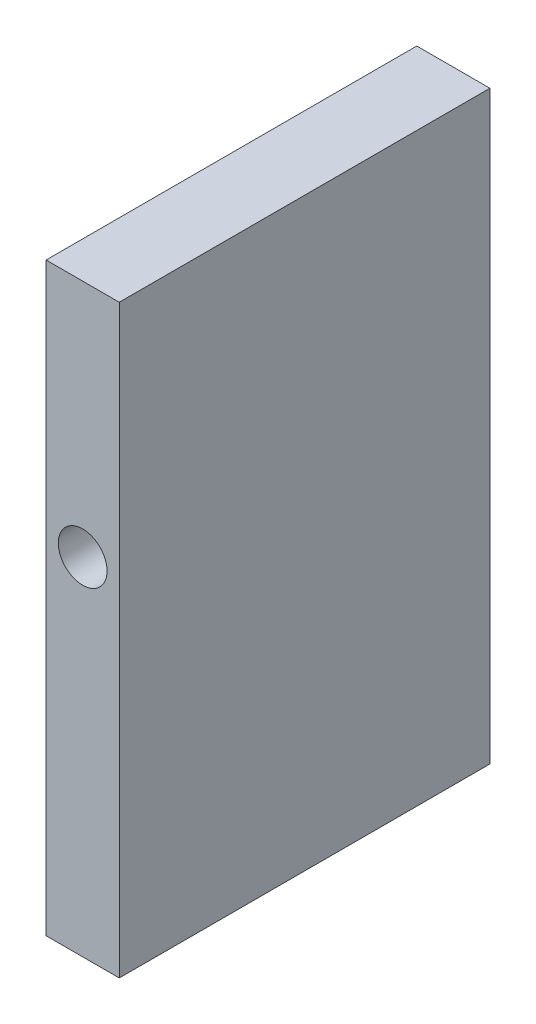
SolidWorks part; units mm, degrees
material "Q235A"
ref_plane "Front Plane" through (0, 0, 0) normal (0, 0, 1) x (1, 0, 0)
ref_plane "Top Plane" through (0, 0, 0) normal (0, 1, 0) x (1, 0, 0)
ref_plane "Right Plane" through (0, 0, 0) normal (1, 0, 0) x (0, 0, -1)
sketch "Sketch1" plane through (0, 0, 0) normal (0, 0, 1) x (1, 0, 0)
  line L1 (7.5, -60) -> (-7.5, -60)
  line L2 (7.5, -60) -> (7.5, 60)
  line L3 (7.5, 60) -> (-7.5, 60)
  line L4 (-7.5, -60) -> (-7.5, 60)
  line L5 (7.5, -60) -> (-7.5, 60) construction
  line L6 (7.5, 60) -> (-7.5, -60) construction
  point P0 (0, 0)
  dimension "D1" = 15
  dimension "D2" = 120
extrude "Boss-Extrude1" add sketch "Sketch1" along normal blind 76
sketch "Sketch2" plane through (0, 0, 76) normal (0, 0, 1) x (1, 0, 0)
  line L0 (7.5, 60) -> (-7.5, 60) construction
  circle A0 centre (0, 11) radius 5
  dimension "D1" = 10
  dimension "D2" = 49
extrude "Cut-Extrude2" cut sketch "Sketch2" against normal through all
